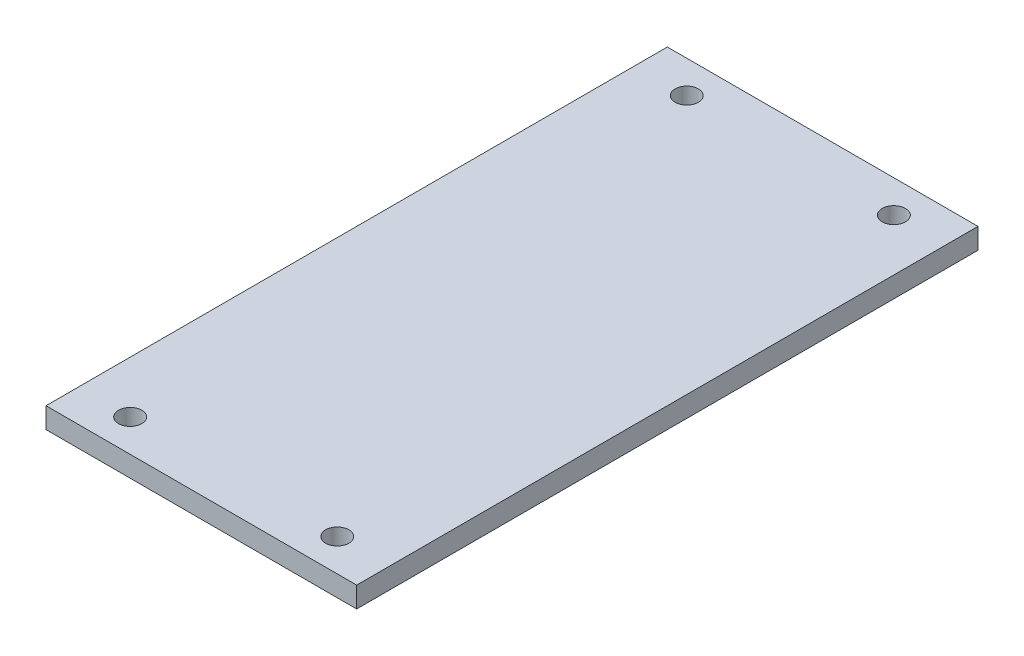
SolidWorks part; units mm, degrees
material "Q235B"
ref_plane "Front Plane" through (0, 0, 0) normal (0, 0, 1) x (1, 0, 0)
ref_plane "Top Plane" through (0, 0, 0) normal (0, 1, 0) x (1, 0, 0)
ref_plane "Right Plane" through (0, 0, 0) normal (1, 0, 0) x (0, 0, -1)
sketch "Sketch1" plane through (0, 0, 0) normal (0, 1, 0) x (1, 0, 0)
  line L1 (120, -240) -> (-120, -240)
  line L2 (120, -240) -> (120, 240)
  line L3 (120, 240) -> (-120, 240)
  line L4 (-120, -240) -> (-120, 240)
  line L5 (120, -240) -> (-120, 240) construction
  line L6 (120, 240) -> (-120, -240) construction
  point P0 (0, 0)
  dimension "D1" = 240
  dimension "D2" = 480
extrude "Boss-Extrude1" add sketch "Sketch1" along normal blind 16
hole_wizard "Ø18.0 (18) Diameter Hole1" positions "Sketch2" profile "Sketch3" hole size "Ø18.0" standard "GB" end condition up to next
sketch "Sketch2" plane through (0, 16, 0) normal (0, 1, 0) x (1, 0, 0)
  line L0 (-80, -215) -> (80, -215) construction
  line L1 (-80, -215) -> (-80, 215) construction
  line L2 (0, 0) -> (0, -215) construction
  line L4 (0, 0) -> (-80, 0) construction
  point P0 (-80, -215)
  point P8 (80, -215)
  point P9 (80, 215)
  point P10 (-80, 215)
  dimension "D3" = 90
  dimension "D4" = 160
  dimension "D5" = 430
  dimension "D1" = 2
  dimension "D2" = 2
sketch "Sketch3" plane through (-80, 16, 215) normal (1, 0, 0) x (0, 0, 1)
  line L0 (0, 0) -> (0, 16)
  line L1 (0, 16) -> (9, 16)
  line L2 (9, 16) -> (9, 0)
  line L5 (9, 0) -> (0, 0)
  line L11 (0, -6.35) -> (0, 107.95) construction
  dimension "通孔孔直径" = 18
  dimension "通孔孔深度" = 16
chamfer "Chamfer1" [suppressed] distance 10 angle 45
fillet "Fillet1" [suppressed] radius 10
